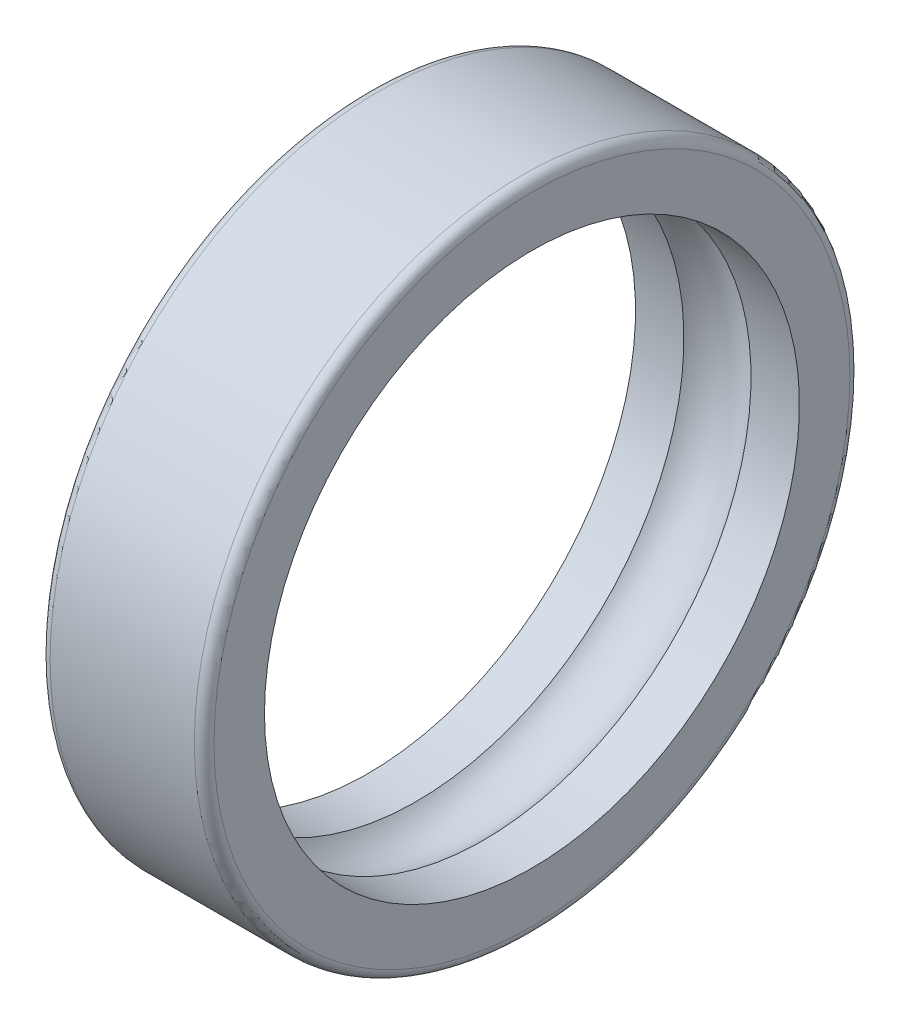
SolidWorks part; units mm, degrees
ref_plane "Front Plane" through (0, 0, 0) normal (0, 0, 1) x (1, 0, 0)
ref_plane "Top Plane" through (0, 0, 0) normal (0, 1, 0) x (1, 0, 0)
ref_plane "Right Plane" through (0, 0, 0) normal (1, 0, 0) x (0, 0, -1)
other "Configuration Table"
sketch "Sketch1" plane through (0, 0, 0) normal (0, 0, 1) x (1, 0, 0)
  line L0 (-5.8509, 0) -> (8.3232, 0) construction
  line L1 (0, 0) -> (0, 67.3748) construction
  line L2 (5.1205, 40.8) -> (12.5, 40.8)
  line L3 (-12.5, 50) -> (12.5, 50)
  line L4 (-12.5, 50) -> (-12.5, 40.8)
  line L5 (-12.5, 40.8) -> (-5.1205, 40.8)
  line L6 (12.5, 50) -> (12.5, 40.8)
  line L7 (-12.5, 50) -> (12.5, 40.8) construction
  line L8 (-12.5, 40.8) -> (12.5, 50) construction
  arc A0 (5.1205, 40.8) -> (-5.1205, 40.8) centre (0, 36.25) ccw
  point P5 (0, 45.4)
  dimension "D4" = 13.7
  dimension "D1" = 9.2
  dimension "D2" = 25
  dimension "D3" = 50
  dimension "D5" = 36.25
revolve "Revolve1" add sketch "Sketch1" angle 360 about L0
fillet "Fillet1" radius 1.5 2 edges at (-12.5, 0, 50) (12.5, 0, 50)
